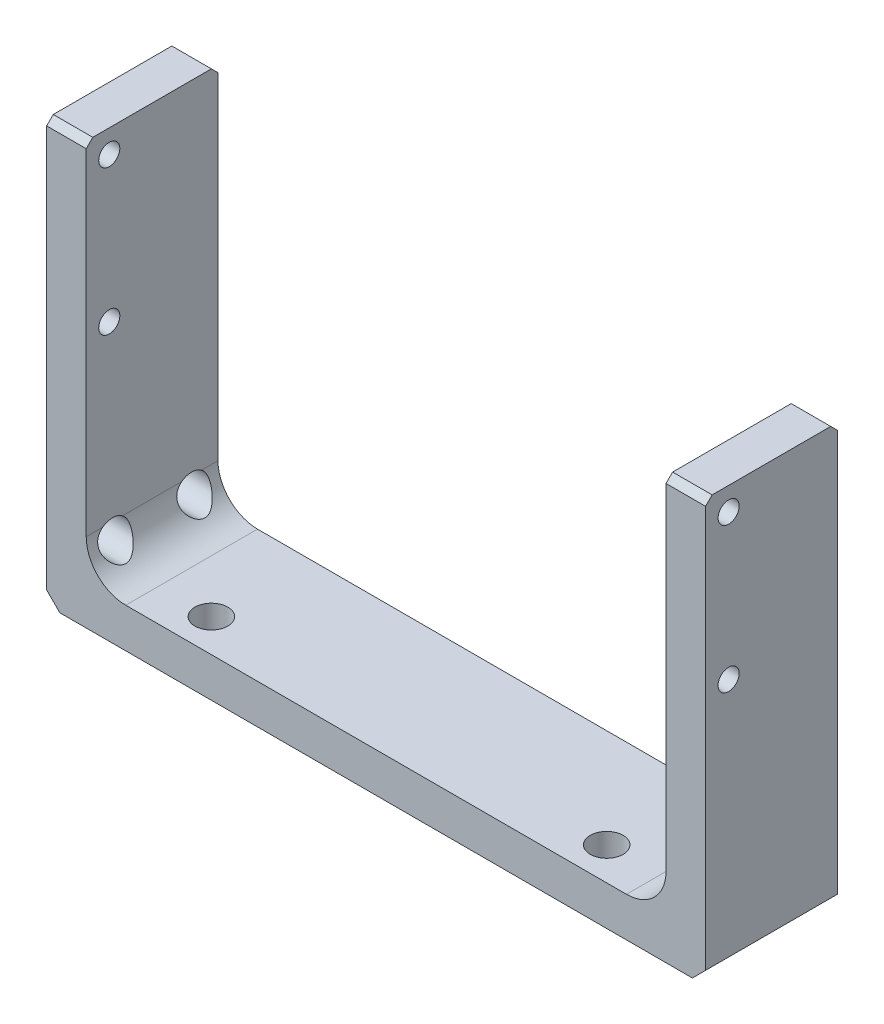
SolidWorks part; units mm, degrees
ref_plane "Front Plane" through (0, 0, 0) normal (0, 0, 1) x (1, 0, 0)
ref_plane "Top Plane" through (0, 0, 0) normal (0, 1, 0) x (1, 0, 0)
ref_plane "Right Plane" through (0, 0, 0) normal (1, 0, 0) x (0, 0, -1)
sketch "Sketch26" plane through (0, 0, 0) normal (0, 0, 1) x (1, 0, 0)
  line L1 (-25, 16) -> (25, 16)
  line L2 (-25, 16) -> (-25, -16)
  line L3 (-25, -16) -> (25, -16)
  line L4 (25, 16) -> (25, -16)
  line L5 (-25, 16) -> (25, -16) construction
  line L6 (-25, -16) -> (25, 16) construction
  point P0 (0, 0)
  dimension "D1" = 50
  dimension "D2" = 32
extrude "Boss-Extrude2" add sketch "Sketch26" along normal mid plane 10
sketch "Sketch27" plane through (0, 0, 5) normal (0, 0, 1) x (1, 0, 0)
  line L0 (25, 16) -> (-25, 16) construction
  line L1 (-22, 16) -> (22, 16)
  line L2 (-22, 16) -> (-22, -13)
  line L3 (-22, -13) -> (22, -13)
  line L4 (22, 16) -> (22, -13)
  line L5 (-22, 16) -> (22, -13) construction
  line L6 (-22, -13) -> (22, 16) construction
  line L7 (-25, 16) -> (-25, -16) construction
  point P0 (0, 1.5)
  dimension "D1" = 3
  dimension "D2" = 29
extrude "Cut-Extrude5" cut sketch "Sketch27" against normal through all
fillet "Fillet1" radius 3 2 edges at (22, -13, 0) (-22, -13, 0)
chamfer "Chamfer1" distance 0.5 angle 45 4 edges at (23.5, 16, 5) (23.5, 16, -5) (-23.5, 16, -5) (-23.5, 16, 5)
chamfer "Chamfer2" distance 1 angle 45 2 edges at (-25, -16, 0) (25, -16, 0)
hole_wizard "M2 Tapped Hole1" positions "Sketch31" profile "Sketch30" tap size "M2" standard "Gb" end condition through all
sketch "Sketch31" plane through (25, 0, 0) normal (1, 0, 0) x (0, 0, -1)
  line L0 (-5, -15) -> (-5, 15.5) construction
  line L1 (-4.5, 16) -> (4.5, 16) construction
  point P0 (-3.25, 14.25)
  point P3 (-3.25, 3.25)
  dimension "D1" = 1.75
  dimension "D2" = 1.75
  dimension "D3" = 11
sketch "Sketch30" plane through (25, 14.25, 3.25) normal (0, 1, 0) x (0, 0, -1)
  line L0 (0, 0) -> (0, 50)
  line L1 (0, 50) -> (0.8, 50)
  line L2 (0.8, 50) -> (0.8, 0)
  line L5 (0.8, 0) -> (0, 0)
  line L11 (0, -6.35) -> (0, 107.95) construction
  dimension "通孔螺纹孔钻头直径" = 1.6
  dimension "通孔螺纹孔钻头深度" = 50
cosmetic thread "Hole Thread1" parameters "D2"=2
cosmetic thread "Hole Thread2" parameters "D2"=2
hole_wizard "Ø2.5 (2.5) Diameter Hole1" positions "Sketch35" profile "Sketch34" hole size "Ø2.5" standard "Gb" end condition through all
sketch "Sketch35" plane through (0, -16, 0) normal (0, -1, 0) x (-1, 0, 0)
  line L0 (25, 5) -> (25, -5) construction
  line L1 (-25, -5) -> (-25, 5) construction
  line L2 (24, -5) -> (-24, -5) construction
  point P0 (15, -2.5)
  point P2 (-15, -2.5)
  dimension "D1" = 10
  dimension "D2" = 10
  dimension "D3" = 2.5
sketch "Sketch34" plane through (-15, -16, 2.5) normal (1, 0, 0) x (0, 0, -1)
  line L0 (0, 0) -> (0, 32)
  line L1 (0, 32) -> (1.25, 32)
  line L2 (1.25, 32) -> (1.25, 0)
  line L5 (1.25, 0) -> (0, 0)
  line L11 (0, -6.35) -> (0, 107.95) construction
  dimension "通孔孔直径" = 2.5
  dimension "通孔孔深度" = 32
hole_wizard "M3 Tapped Hole2" positions "Sketch37" profile "Sketch36" tap size "M3" standard "Gb"
sketch "Sketch37" plane through (-25, 0, 0) normal (-1, 0, 0) x (0, 0, 1)
  line L0 (0, 0) -> (0, -17.683) construction
  line L2 (5, -16) -> (-5, -16) construction
  point P0 (-3, -11)
  point P2 (3, -11)
  dimension "D1" = 6
  dimension "D2" = 5
sketch "Sketch36" plane through (-25, -11, -3) normal (0, 1, 0) x (0, 0, 1)
  line L0 (0, 0) -> (0, 3.1716)
  line L1 (0, 3.1716) -> (1.25, 3.1716)
  line L2 (1.25, 3.1716) -> (1.25, 0)
  line L5 (1.25, 0) -> (0, 0)
  line L11 (0, -6.35) -> (0, 107.95) construction
  dimension "通孔螺纹孔钻头直径" = 2.5
  dimension "通孔螺纹孔钻头深度" = 3.1716
cosmetic thread "Hole Thread4" parameters "D2"=3
cosmetic thread "Hole Thread5" parameters "D2"=3
